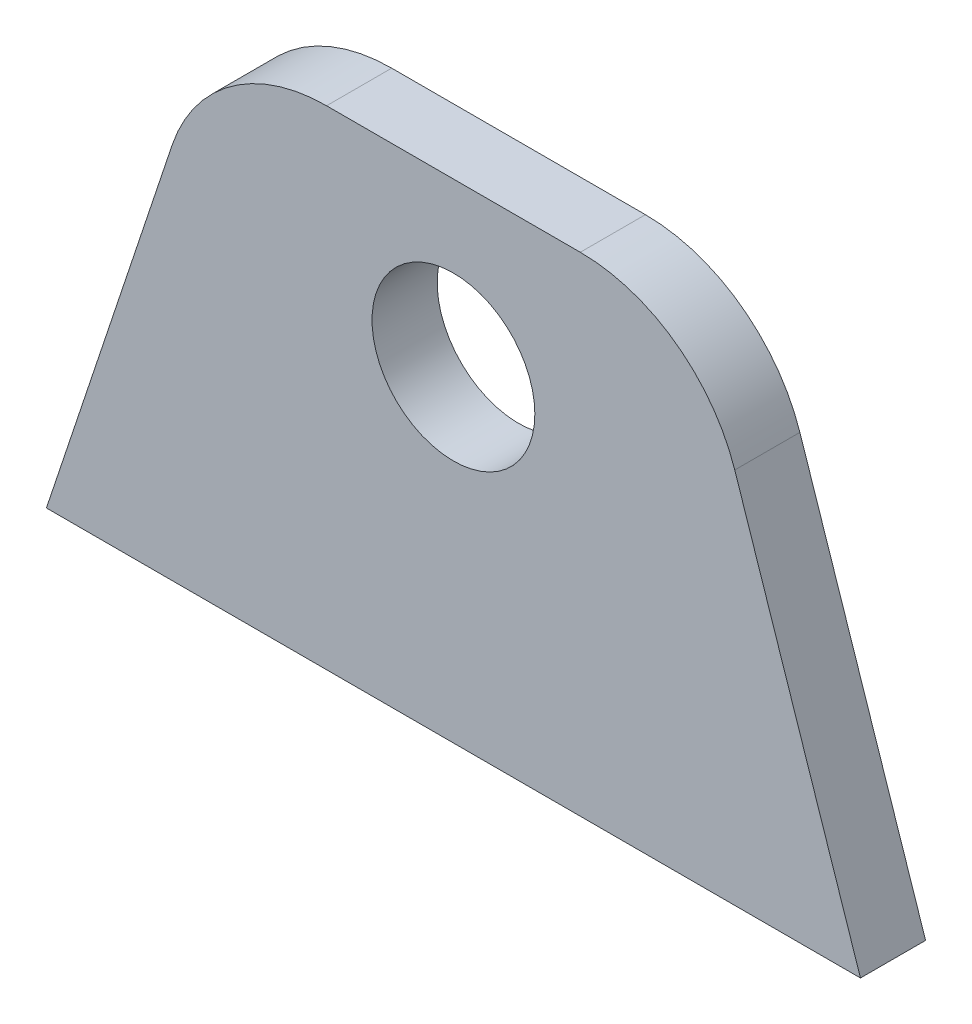
from build123d import *

# Parameters (mm, degrees)
SKETCH1_R           = 5
BOSS_EXTRUDE1_DEPTH = 4


with BuildPart() as part:
    # Sketch1 → Boss-Extrude1 (new body)
    with BuildSketch(Plane.XY):
        with BuildLine():
            Line((0, 0), (50, 0))
            Line((50, 0), (42.27924078, 23.16227766))
            ThreePointArc((42.27924078, 23.16227766), (38.639510646, 28.112421852), (32.792407799, 30))
            Line((32.792407799, 30), (17.207592201, 30))
            ThreePointArc((17.207592201, 30), (11.360489354, 28.112421852), (7.72075922, 23.16227766))
            Line((7.72075922, 23.16227766), (0, 0))
        make_face()
        with Locations((25, 20)):
            Circle(SKETCH1_R, mode=Mode.SUBTRACT)
    extrude(amount=BOSS_EXTRUDE1_DEPTH)


solid = part.part
